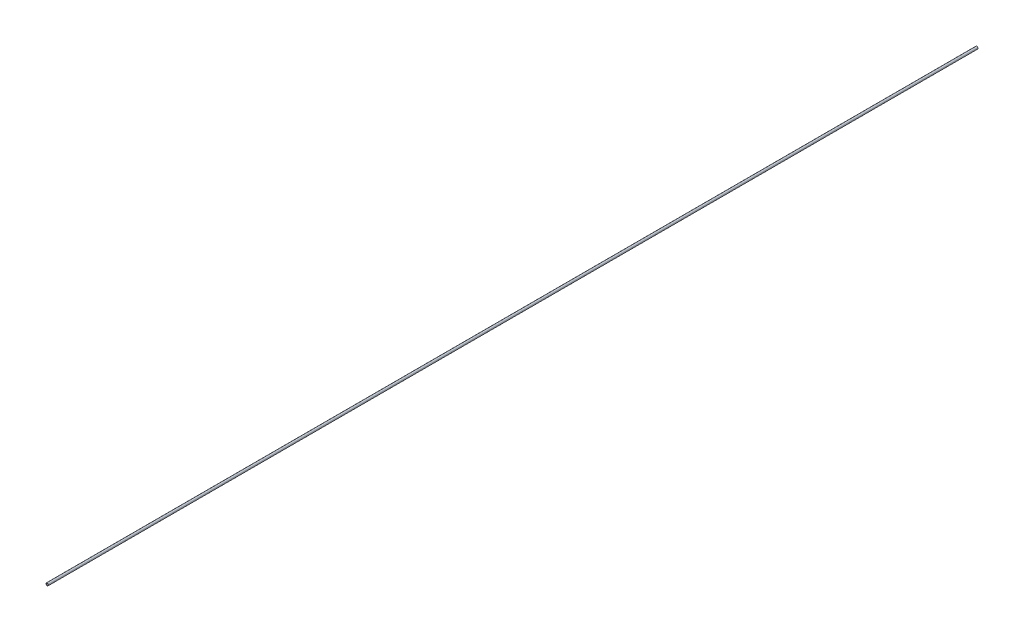
SolidWorks part; units mm, degrees
material "普通碳钢"
ref_plane "Front Plane" through (0, 0, 0) normal (0, 0, 1) x (1, 0, 0)
ref_plane "Top Plane" through (0, 0, 0) normal (0, 1, 0) x (1, 0, 0)
ref_plane "Right Plane" through (0, 0, 0) normal (1, 0, 0) x (0, 0, -1)
sketch "Sketch1" plane through (0, 0, 0) normal (0, 0, 1) x (1, 0, 0)
  circle A0 centre (0, 0) radius 9.525
  circle A1 centre (0, 0) radius 6.775
  dimension "D1" = 19.05
  dimension "D2" = 2.75
extrude "Boss-Extrude1" add sketch "Sketch1" along normal mid plane 7329
